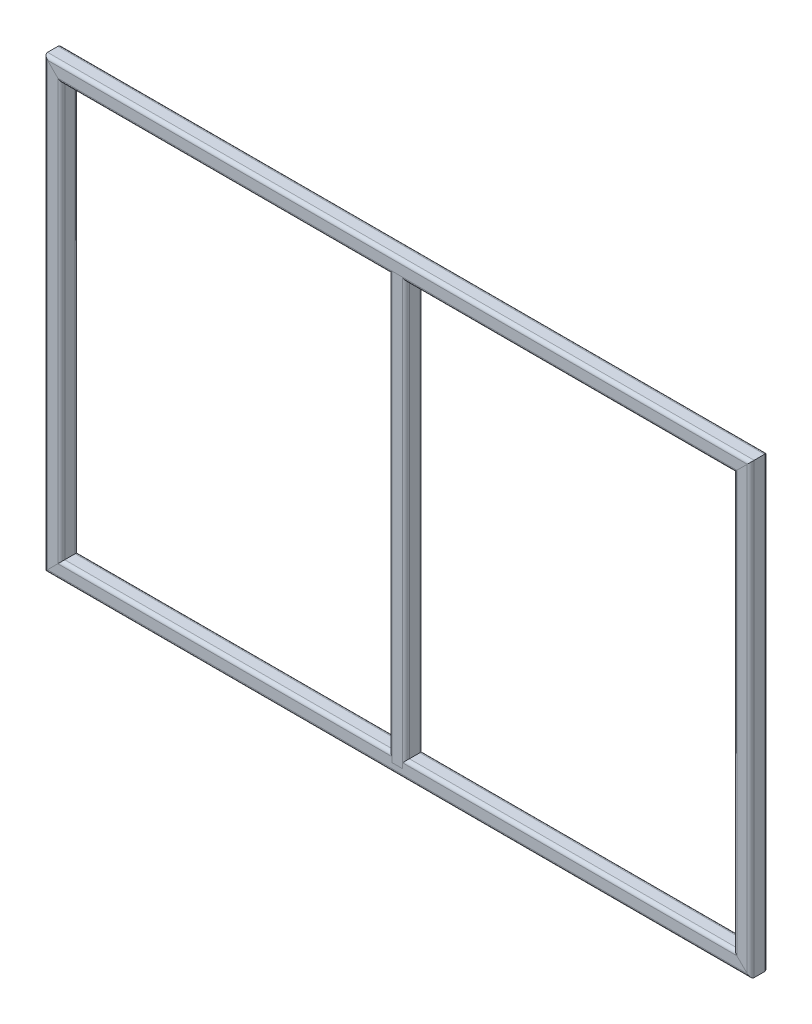
SolidWorks part; units mm, degrees
ref_plane "Front Plane" through (0, 0, 0) normal (0, 0, 1) x (1, 0, 0)
ref_plane "Top Plane" through (0, 0, 0) normal (0, 1, 0) x (1, 0, 0)
ref_plane "Right Plane" through (0, 0, 0) normal (1, 0, 0) x (0, 0, -1)
sketch "草图1" plane through (0, 0, 0) normal (0, 0, 1) x (1, 0, 0)
  line L0 (0, 250) -> (0, -250)
  line L1 (-400, 250) -> (400, 250)
  line L2 (-400, 250) -> (-400, -250)
  line L3 (-400, -250) -> (400, -250)
  line L4 (400, 250) -> (400, -250)
  line L5 (-400, 250) -> (400, -250) construction
  line L6 (-400, -250) -> (400, 250) construction
  point P0 (0, 0)
  dimension "D1" = 800
  dimension "D2" = 500
sketch "Sketch2" plane through (0, 0, 0) normal (0, 0, 1) x (1, 0, 0)
other "Square tube 20 X 20 X 2(1)"
ref_plane "Plane4" through (-400, 250, 0) normal (1, 0, 0) x (0, 1, 0)
sketch "Sketch1" plane through (-400, 250, 0) normal (1, 0, 0) x (0, 1, 0)
  line L0 (-6, -8) -> (6, -8)
  line L1 (-8, -6) -> (-8, 6)
  line L2 (6, 8) -> (-6, 8)
  line L3 (8, 6) -> (8, -6)
  line L4 (-6, -10) -> (6, -10)
  line L5 (-10, -6) -> (-10, 6)
  line L6 (6, 10) -> (-6, 10)
  line L7 (10, 6) -> (10, -6)
  arc A0 (10, 6) -> (6, 10) centre (6, 6) ccw
  arc A1 (6, -10) -> (10, -6) centre (6, -6) ccw
  arc A2 (-10, -6) -> (-6, -10) centre (-6, -6) ccw
  arc A3 (-6, 10) -> (-10, 6) centre (-6, 6) ccw
  arc A4 (-6, 8) -> (-8, 6) centre (-6, 6) ccw
  arc A5 (8, 6) -> (6, 8) centre (6, 6) ccw
  arc A6 (6, -8) -> (8, -6) centre (6, -6) ccw
  arc A7 (-8, -6) -> (-6, -8) centre (-6, -6) ccw
  point P0 (-10, 0)
  point P1 (10, 0)
  point P2 (0, 10)
  point P3 (0, -10)
  point P4 (0, 0)
  point P5 (-10, -10)
  point P6 (10, -10)
  point P7 (10, 10)
  point P8 (-10, 10)
  point P33 (0, 0)
  dimension "D1" = 4
  dimension "Thickness" = 2
  dimension "V_leg" = 20
other "Square tube 20 X 20 X 2(2)"
ref_plane "Plane5" through (0, 250, 0) normal (0, -1, 0) x (1, 0, 0)
sketch "Sketch11" plane through (0, 250, 0) normal (0, -1, 0) x (1, 0, 0)
  line L0 (-6, -8) -> (6, -8)
  line L1 (-8, -6) -> (-8, 6)
  line L2 (6, 8) -> (-6, 8)
  line L3 (8, 6) -> (8, -6)
  line L4 (-6, -10) -> (6, -10)
  line L5 (-10, -6) -> (-10, 6)
  line L6 (6, 10) -> (-6, 10)
  line L7 (10, 6) -> (10, -6)
  arc A0 (10, 6) -> (6, 10) centre (6, 6) ccw
  arc A1 (6, -10) -> (10, -6) centre (6, -6) ccw
  arc A2 (-10, -6) -> (-6, -10) centre (-6, -6) ccw
  arc A3 (-6, 10) -> (-10, 6) centre (-6, 6) ccw
  arc A4 (-6, 8) -> (-8, 6) centre (-6, 6) ccw
  arc A5 (8, 6) -> (6, 8) centre (6, 6) ccw
  arc A6 (6, -8) -> (8, -6) centre (6, -6) ccw
  arc A7 (-8, -6) -> (-6, -8) centre (-6, -6) ccw
  point P0 (-10, 0)
  point P1 (10, 0)
  point P2 (0, 10)
  point P3 (0, -10)
  point P4 (0, 0)
  point P5 (-10, -10)
  point P6 (10, -10)
  point P7 (10, 10)
  point P8 (-10, 10)
  point P33 (0, 0)
  dimension "D1" = 4
  dimension "Thickness" = 2
  dimension "V_leg" = 20
